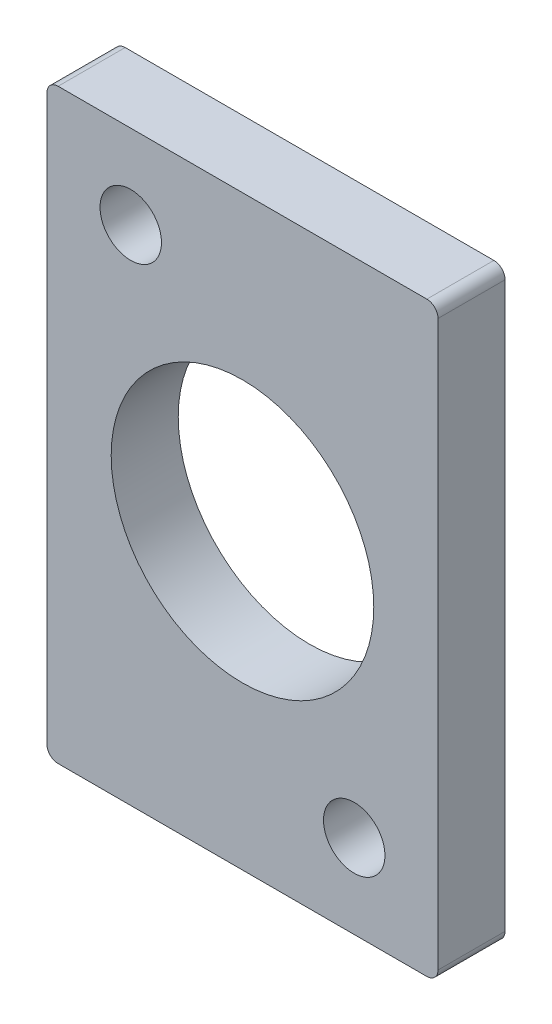
from build123d import *

# Parameters (mm, degrees)
SKETCH_1_R      = 23.5
SKETCH_1_R_2    = 5.5
EXTRUDE_1_DEPTH = 12


with BuildPart() as part:
    # 草图1 → 凸台-拉伸1 (new body)
    with BuildSketch(Plane.XY):
        with BuildLine():
            Line((-33, 52.5), (33, 52.5))
            ThreePointArc((33, 52.5), (34.414213562, 51.914213562), (35, 50.5))
            Line((35, 50.5), (35, -50.5))
            ThreePointArc((35, -50.5), (34.414213562, -51.914213562), (33, -52.5))
            Line((33, -52.5), (-33, -52.5))
            ThreePointArc((-33, -52.5), (-34.414213562, -51.914213562), (-35, -50.5))
            Line((-35, -50.5), (-35, 50.5))
            ThreePointArc((-35, 50.5), (-34.414213562, 51.914213562), (-33, 52.5))
        make_face()
        Circle(SKETCH_1_R, mode=Mode.SUBTRACT)
        with Locations((-20, 37.5)):
            Circle(SKETCH_1_R_2, mode=Mode.SUBTRACT)
        with Locations((20, -37.5)):
            Circle(SKETCH_1_R_2, mode=Mode.SUBTRACT)
    extrude(amount=EXTRUDE_1_DEPTH)


solid = part.part
